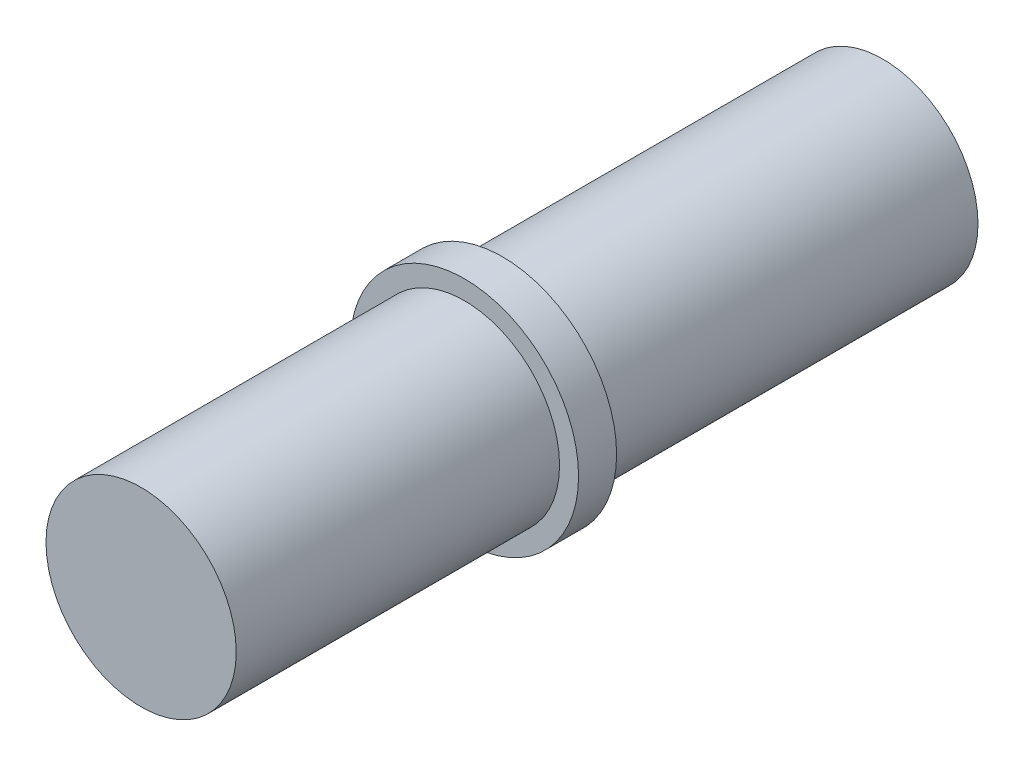
SolidWorks part; units mm, degrees
material "AISI 1045 钢，冷拔"
ref_plane "前视基准面" through (0, 0, 0) normal (0, 0, 1) x (1, 0, 0)
ref_plane "上视基准面" through (0, 0, 0) normal (0, 1, 0) x (1, 0, 0)
ref_plane "右视基准面" through (0, 0, 0) normal (1, 0, 0) x (0, 0, -1)
other "Configuration Table"
sketch "草图1" plane through (0, 0, 0) normal (0, 0, 1) x (1, 0, 0)
  circle A0 centre (0, 0) radius 7.5
  dimension "D1" = 15
extrude "凸台-拉伸1" add sketch "草图1" along normal blind 100
sketch "草图2" plane through (0, 0, 100) normal (0, 0, 1) x (1, 0, 0)
  circle A0 centre (0, 0) radius 9
  dimension "D1" = 18
extrude "凸台-拉伸2" add sketch "草图2" against normal blind 3 from offset 25.5 offset against normal yes
sketch "草图3" plane through (0, 0, 0) normal (0, 0, -1) x (-1, 0, 0)
  circle A0 centre (0, 0) radius 9
  dimension "D1" = 18
extrude "凸台-拉伸3" add sketch "草图3" against normal blind 3 from offset 25.5 offset against normal yes
sketch "草图4" plane through (0, 0, 0) normal (0, 0, -1) x (-1, 0, 0)
  circle A0 centre (0, 0) radius 7.5
extrude "凸台-拉伸4" add sketch "草图4" along normal blind 40
sketch "草图5" plane through (0, 0, -40) normal (0, 0, -1) x (-1, 0, 0)
  circle A0 centre (0, 0) radius 10
  dimension "D1" = 20
extrude "切除-拉伸2" cut sketch "草图5" against normal blind 81.5
